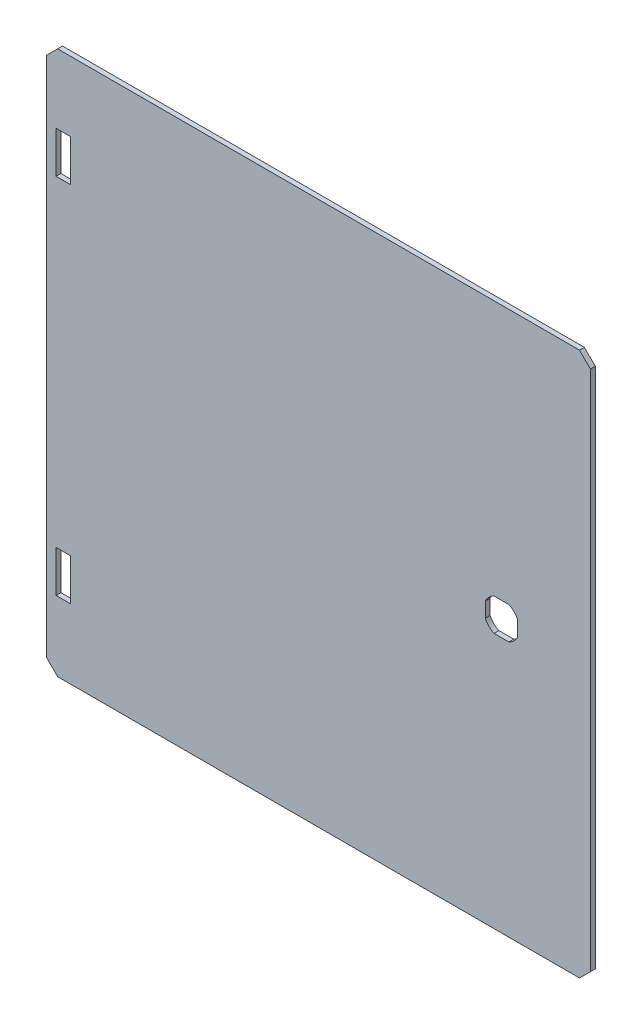
SolidWorks part; units mm, degrees
ref_plane "Front Plane" through (0, 0, 0) normal (0, 0, 1) x (1, 0, 0)
ref_plane "Top Plane" through (0, 0, 0) normal (0, 1, 0) x (1, 0, 0)
ref_plane "Right Plane" through (0, 0, 0) normal (1, 0, 0) x (0, 0, -1)
other "Configuration Table"
sketch "Sketch1" plane through (0, 0, 0) normal (0, 0, 1) x (1, 0, 0)
  line L0 (108.4174, 10) -> (117.5826, 10)
  line L1 (-162.2, 125) -> (-153.2, 125)
  line L2 (-162.2, 125) -> (-162.2, 99.3)
  line L3 (-162.2, 99.3) -> (-153.2, 99.3)
  line L4 (-153.2, 125) -> (-153.2, 99.3)
  line L5 (-162.2, -99.3) -> (-153.2, -99.3)
  line L6 (-162.2, -99.3) -> (-162.2, -125)
  line L7 (-162.2, -125) -> (-153.2, -125)
  line L16 (165, -160) -> (165, 160)
  line L17 (165, 160) -> (160, 165)
  line L18 (160, 165) -> (-160, 165)
  line L19 (-160, 165) -> (-165, 160)
  line L20 (-165, 160) -> (-165, -160)
  line L21 (-165, -160) -> (-160, -165)
  line L22 (-160, -165) -> (160, -165)
  line L23 (160, -165) -> (165, -160)
  line L24 (-153.2, -99.3) -> (-153.2, -125)
  line L25 (103, 4.5826) -> (103, -4.5826)
  line L26 (108.4174, -10) -> (117.5826, -10)
  line L27 (123, 4.5826) -> (123, -4.5826)
  arc A0 (108.4174, 10) -> (103, 4.5826) centre (113, 0) ccw
  arc A1 (103, -4.5826) -> (108.4174, -10) centre (113, 0) ccw
  arc A2 (117.5826, -10) -> (123, -4.5826) centre (113, 0) ccw
  arc A3 (123, 4.5826) -> (117.5826, 10) centre (113, 0) ccw
extrude "Boss-Extrude1" add sketch "Sketch1" along normal blind 3
sketch "Sketch2" plane through (0, 0, 3) normal (0, 0, 1) x (1, 0, 0)
  line L0 (168, -161.2426) -> (168, 161.2426)
  line L1 (168, 161.2426) -> (161.2426, 168)
  line L2 (161.2426, 168) -> (-161.2426, 168)
  line L3 (-161.2426, 168) -> (-168, 161.2426)
  line L4 (-168, 161.2426) -> (-168, -161.2426)
  line L5 (-168, -161.2426) -> (-161.2426, -168)
  line L6 (-161.2426, -168) -> (161.2426, -168)
  line L7 (161.2426, -168) -> (168, -161.2426)
  line L8 (160, -165) -> (165, -160)
  line L9 (165, -160) -> (165, 160)
  line L10 (165, 160) -> (160, 165)
  line L11 (160, 165) -> (-160, 165)
  line L12 (-160, 165) -> (-165, 160)
  line L13 (-165, 160) -> (-165, -160)
  line L14 (-165, -160) -> (-160, -165)
  line L15 (-160, -165) -> (160, -165)
  line L16 (160, -165) -> (165, -160)
  line L17 (165, -160) -> (165, 160)
  line L18 (165, 160) -> (160, 165)
  line L19 (160, 165) -> (-160, 165)
  line L20 (-160, 165) -> (-165, 160)
  line L21 (-165, 160) -> (-165, -160)
  line L22 (-165, -160) -> (-160, -165)
  line L23 (-160, -165) -> (160, -165)
  dimension "D1" = 0
  dimension "D2" = 3
extrude "Boss-Extrude2" add sketch "Sketch2" against normal blind 3
